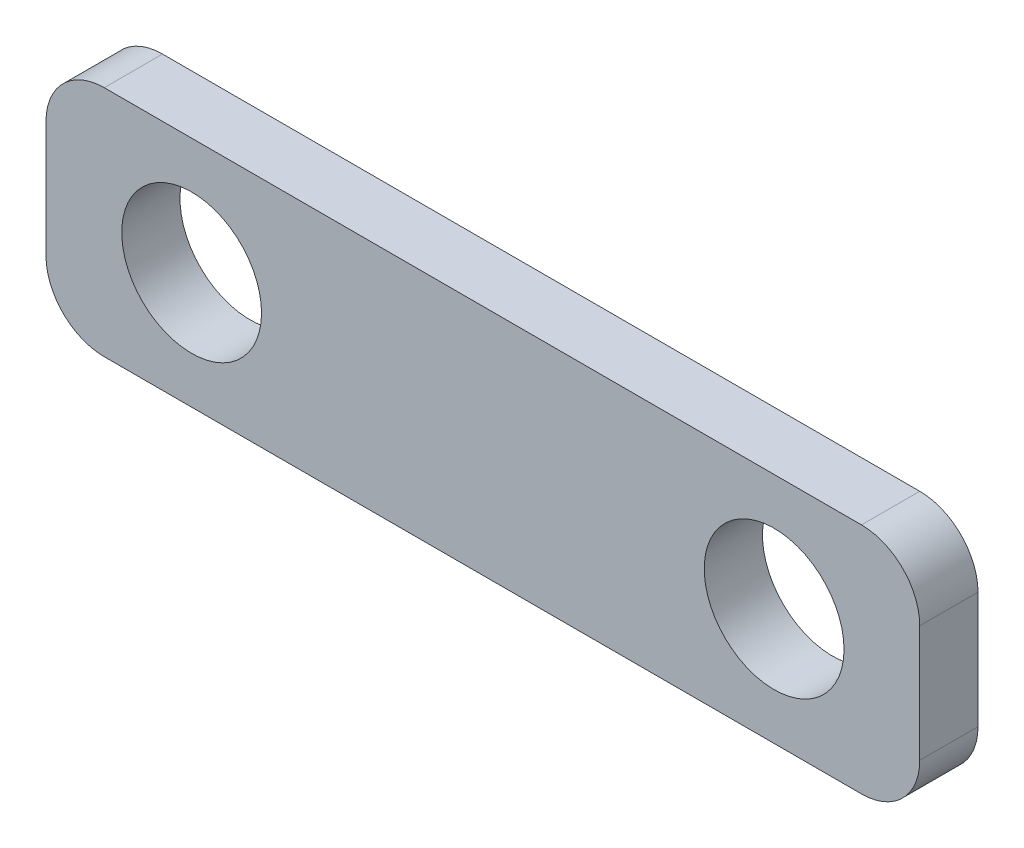
from build123d import *

# Parameters (mm, degrees)
SKETCH1_W           = 150
SKETCH1_H           = 40
SKETCH1_R           = 12
BOSS_EXTRUDE1_DEPTH = 10
FILLET1_R           = 10


with BuildPart() as part:
    # Sketch1 → Boss-Extrude1 (new body)
    with BuildSketch(Plane.XY):
        Rectangle(SKETCH1_W, SKETCH1_H)
        with Locations((50, 0)):
            Circle(SKETCH1_R, mode=Mode.SUBTRACT)
        with Locations((-50, 0)):
            Circle(SKETCH1_R, mode=Mode.SUBTRACT)
    extrude(amount=BOSS_EXTRUDE1_DEPTH)

    # Fillet1
    fillet1_edges = [part.edges().sort_by_distance(p)[0] for p in [
        (75, -20, 5),
        (-75, -20, 5),
        (-75, 20, 5),
        (75, 20, 5),
    ]]
    fillet(fillet1_edges, radius=FILLET1_R)


solid = part.part
